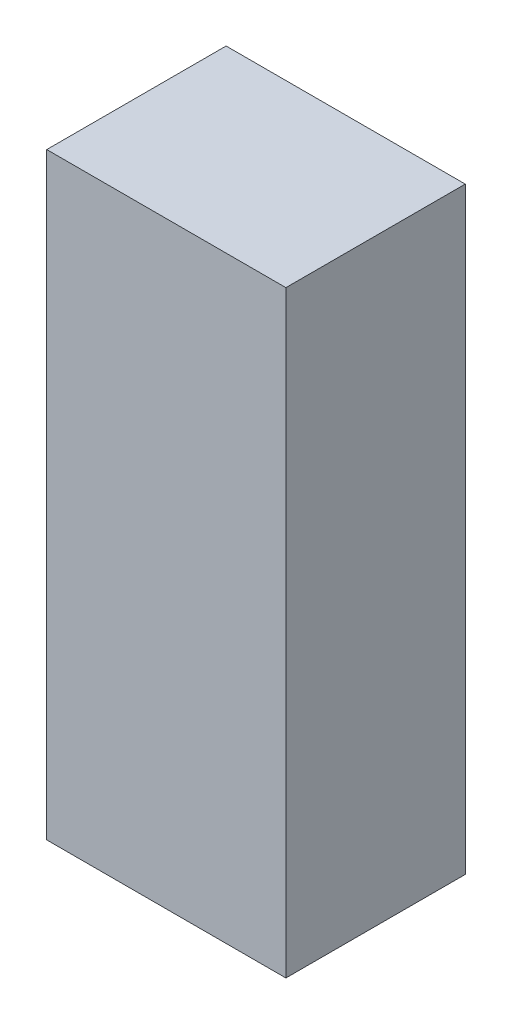
from build123d import *

# Parameters (mm, degrees)
SKETCH1_W           = 20
SKETCH1_H           = 50
BOSS_EXTRUDE1_DEPTH = 15


with BuildPart() as part:
    # Sketch1 → Boss-Extrude1 (new body)
    with BuildSketch(Plane.XY):
        with Locations((10, 25)):
            Rectangle(SKETCH1_W, SKETCH1_H)
    extrude(amount=BOSS_EXTRUDE1_DEPTH)


solid = part.part
